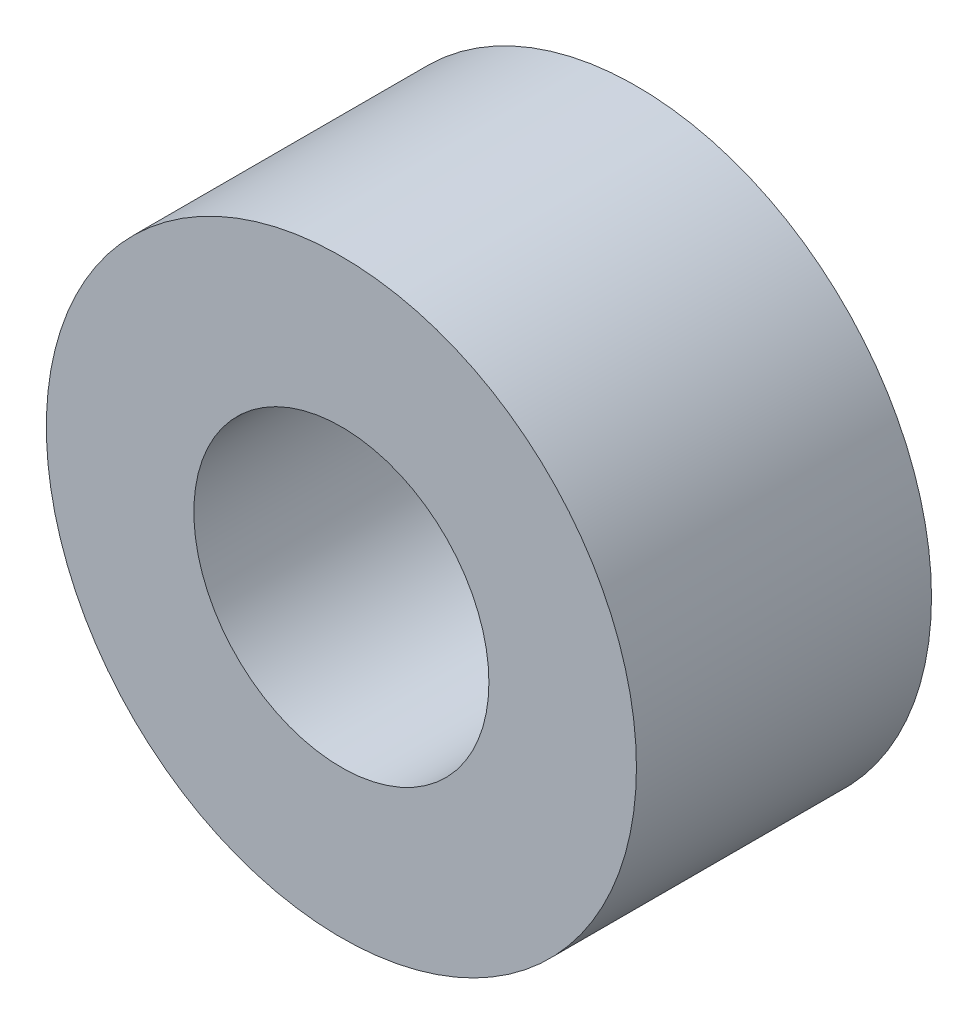
from build123d import *

# Parameters (mm, degrees)
SKETCH_1_R      = 40
SKETCH_1_R_2    = 20
EXTRUDE_1_DEPTH = 20


with BuildPart() as part:
    # 草图1 → 凸台-拉伸1 (new, symmetric)
    with BuildSketch(Plane.XY):
        Circle(SKETCH_1_R)
        Circle(SKETCH_1_R_2, mode=Mode.SUBTRACT)
    extrude(amount=EXTRUDE_1_DEPTH, both=True)


solid = part.part
